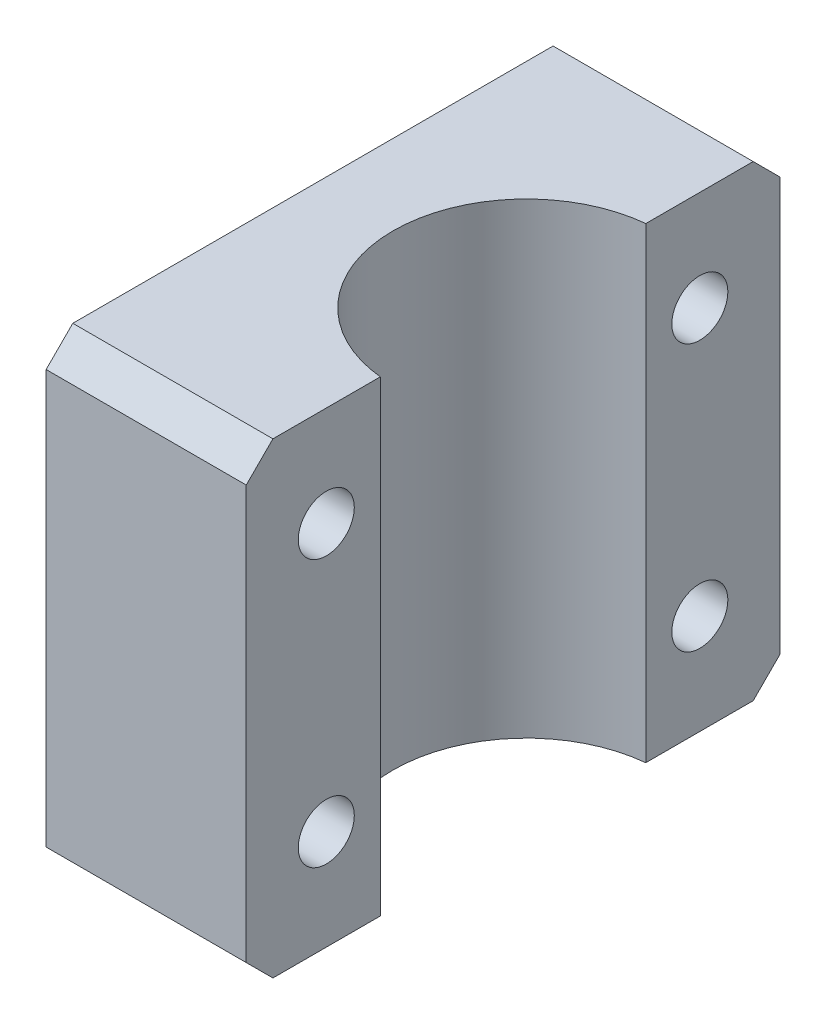
SolidWorks part; units mm, degrees
ref_plane "前视基准面" through (0, 0, 0) normal (0, 0, 1) x (1, 0, 0)
ref_plane "上视基准面" through (0, 0, 0) normal (0, 1, 0) x (1, 0, 0)
ref_plane "右视基准面" through (0, 0, 0) normal (1, 0, 0) x (0, 0, -1)
sketch "草图1" plane through (0, 0, 0) normal (0, 1, 0) x (1, 0, 0)
  line L0 (7.5, 9.9499) -> (7.5, 20)
  line L1 (-7.5, -20) -> (7.5, -20)
  line L2 (-7.5, -20) -> (-7.5, 20)
  line L3 (-7.5, 20) -> (7.5, 20)
  line L4 (7.5, -20) -> (7.5, -9.9499)
  line L5 (-7.5, -20) -> (7.5, 20) construction
  line L6 (-7.5, 20) -> (7.5, -20) construction
  arc A0 (7.5, 9.9499) -> (7.5, -9.9499) centre (8.5, 0) ccw
  point P0 (0, 0)
  dimension "D1" = 20
  dimension "D2" = 1
  dimension "D3" = 40
  dimension "D4" = 15
extrude "凸台-拉伸1" add sketch "草图1" along normal mid plane 35
chamfer "倒角1" distance 2 angle 45 4 edges at (0, -17.5, 20) (0, 17.5, 20) (0, 17.5, -20) (0, -17.5, -20)
sketch "草图4" plane through (7.5, 0, 0) normal (1, 0, 0) x (0, 0, -1)
  point P0 (-14, 10)
  point P3 (14, 10)
  point P6 (14, -10)
  point P9 (-14, -10)
hole_wizard "M5 螺纹孔1" positions "草图4" profile "草图3" tap size "M5" standard "GB" end condition through all
sketch "草图3" plane through (7.5, 10, 14) normal (0, 1, 0) x (0, 0, -1)
  line L0 (0, 0) -> (0, 15)
  line L1 (0, 15) -> (2.1, 15)
  line L2 (2.1, 15) -> (2.1, 0)
  line L5 (2.1, 0) -> (0, 0)
  line L11 (0, -6.35) -> (0, 107.95) construction
  dimension "通孔螺纹孔钻头直径" = 4.2
  dimension "通孔螺纹孔钻头深度" = 15
cosmetic thread "孔螺纹线1"
cosmetic thread "孔螺纹线2"
cosmetic thread "孔螺纹线3"
cosmetic thread "孔螺纹线4"
